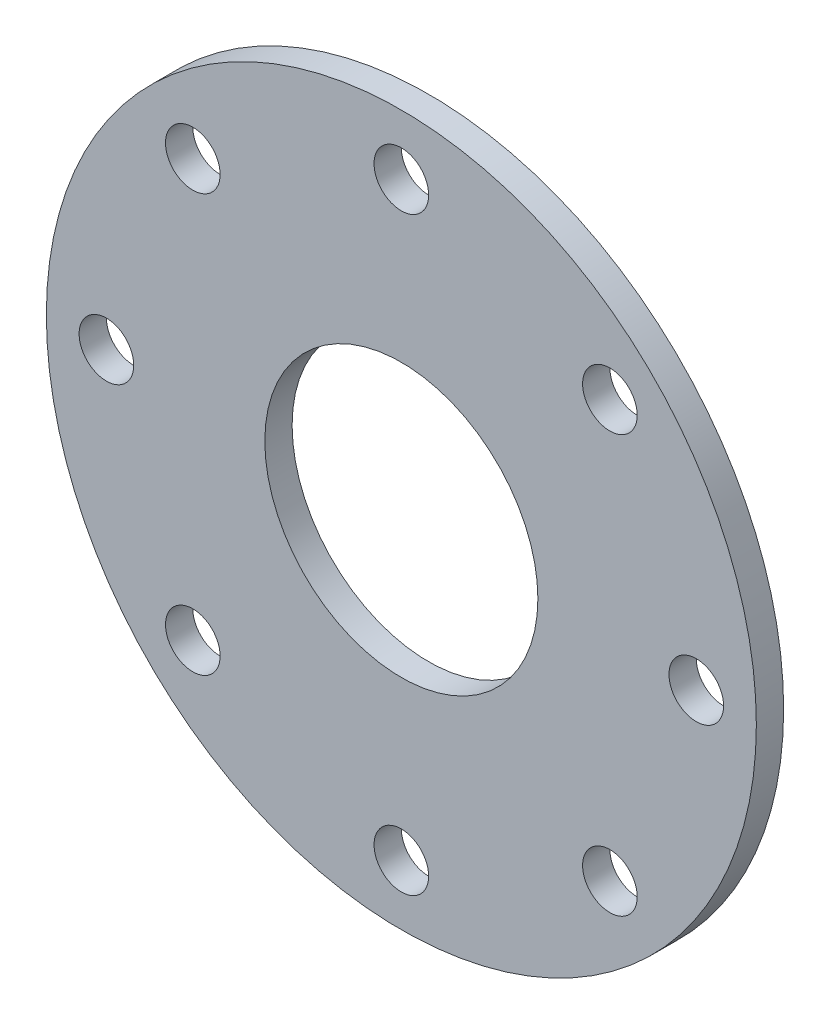
SolidWorks part; units mm, degrees
ref_plane "前视基准面" through (0, 0, 0) normal (0, 0, 1) x (1, 0, 0)
ref_plane "上视基准面" through (0, 0, 0) normal (0, 1, 0) x (1, 0, 0)
ref_plane "右视基准面" through (0, 0, 0) normal (1, 0, 0) x (0, 0, -1)
sketch "草图1" plane through (0, 0, 0) normal (0, 0, 1) x (1, 0, 0)
  circle A0 centre (0, 0) radius 130
  circle A1 centre (0, 0) radius 108 construction
  circle A2 centre (0, 108) radius 10
  circle A3 centre (76.3675, 76.3675) radius 10
  circle A4 centre (108, 0) radius 10
  circle A5 centre (76.3675, -76.3675) radius 10
  circle A6 centre (0, -108) radius 10
  circle A7 centre (-76.3675, -76.3675) radius 10
  circle A8 centre (-108, 0) radius 10
  circle A9 centre (-76.3675, 76.3675) radius 10
  point P22 (0, 0)
  dimension "D1" = 260
  dimension "D2" = 8
extrude "凸台-拉伸1" add sketch "草图1" along normal mid plane 10
sketch "草图2" plane through (0, 0, 5) normal (0, 0, 1) x (1, 0, 0)
  circle A0 centre (0, 0) radius 50
  dimension "D1" = 100
extrude "切除-拉伸1" cut sketch "草图2" against normal blind 10
